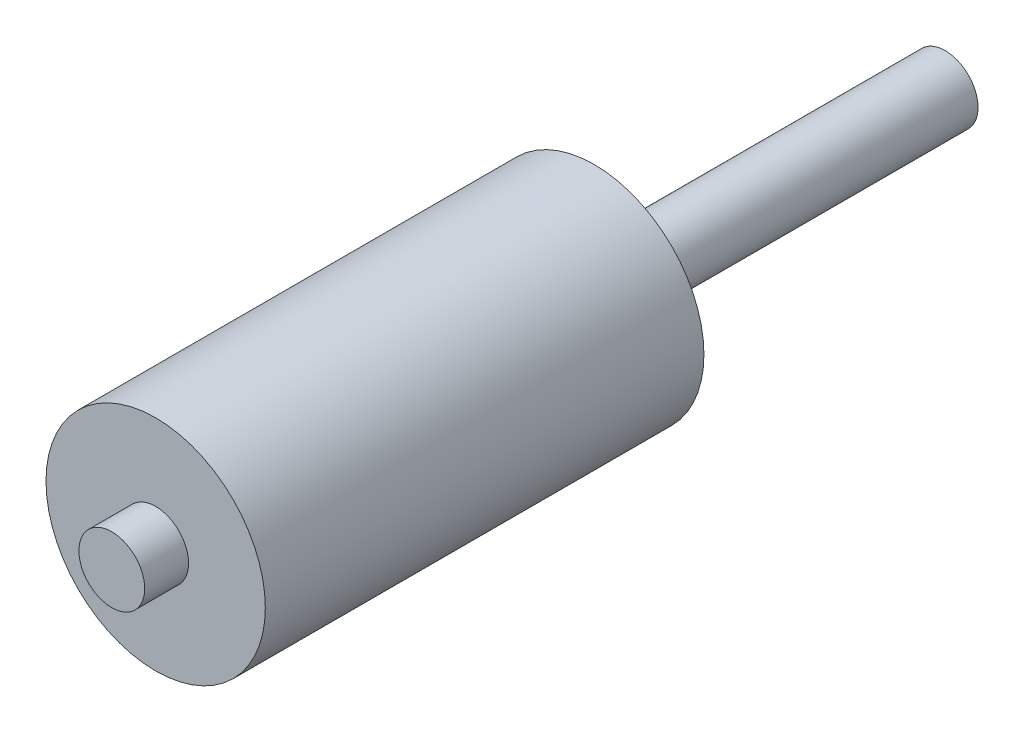
SolidWorks part; units mm, degrees
ref_plane "前视基准面" through (0, 0, 0) normal (0, 0, 1) x (1, 0, 0)
ref_plane "上视基准面" through (0, 0, 0) normal (0, 1, 0) x (1, 0, 0)
ref_plane "右视基准面" through (0, 0, 0) normal (1, 0, 0) x (0, 0, -1)
sketch "草图1" plane through (0, 0, 0) normal (0, 0, 1) x (1, 0, 0)
  circle A0 centre (0, 0) radius 25
  dimension "D1" = 50
extrude "凸台-拉伸1" add sketch "草图1" along normal blind 100
sketch "草图2" plane through (0, 0, 100) normal (0, 0, 1) x (1, 0, 0)
  circle A0 centre (0, 0) radius 7.5
  dimension "D1" = 15
extrude "凸台-拉伸2" add sketch "草图2" along normal blind 10
sketch "草图3" plane through (0, 0, 0) normal (0, 0, -1) x (-1, 0, 0)
  circle A0 centre (0, 0) radius 7.5
  dimension "D1" = 15
extrude "凸台-拉伸3" add sketch "草图3" along normal blind 80
